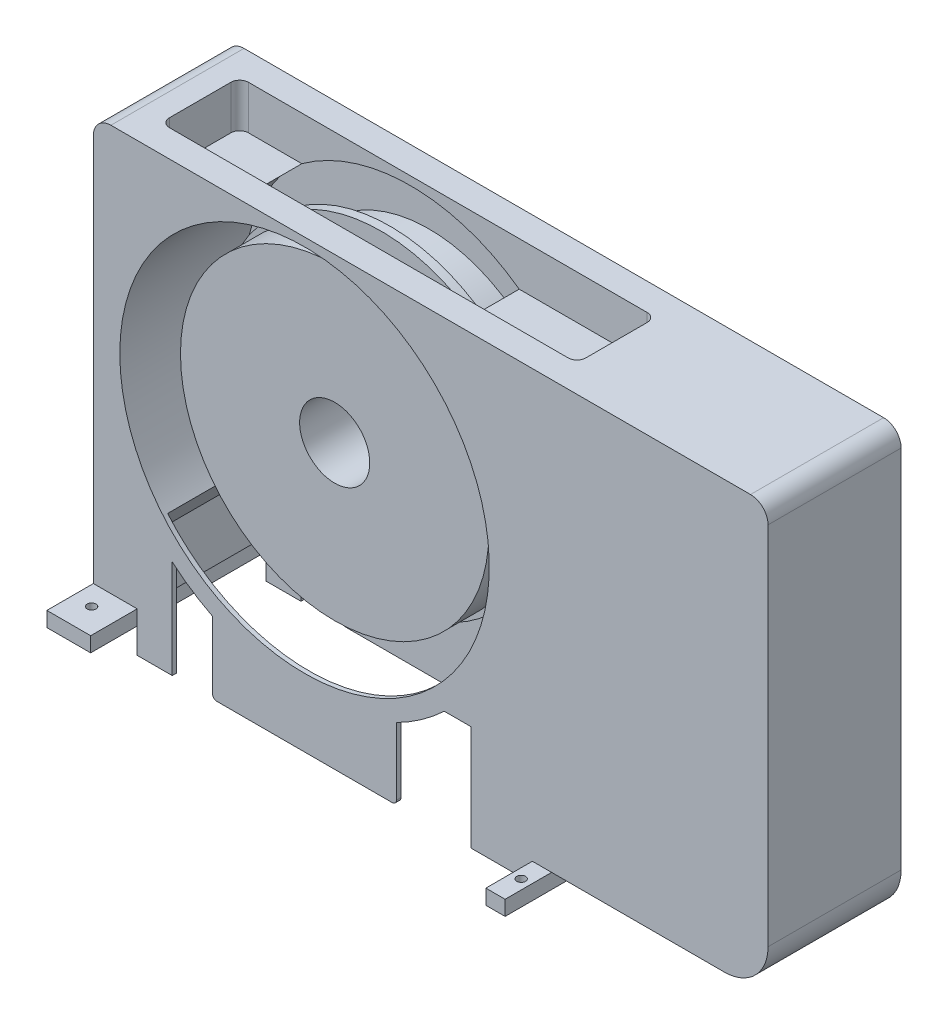
from build123d import *

# Parameters (mm, degrees)
SKETCH2_W             = 50
SKETCH2_H             = 17
BOSS_EXTRUDE1_DEPTH   = 205
SKETCH2_W_2           = 22
BOSS_EXTRUDE1_2_DEPTH = 205
SKETCH3_W             = 237
SKETCH3_H             = 453
BOSS_EXTRUDE2_DEPTH   = 151.9
BOSS_EXTRUDE3_DEPTH   = 10
SKETCH5_W             = 237
SKETCH5_H             = 453
BOSS_EXTRUDE4_DEPTH   = 5
SKETCH6_W             = 237
SKETCH6_H             = 453
BOSS_EXTRUDE5_DEPTH   = 5
BOSS_EXTRUDE7_DEPTH   = 5
BOSS_EXTRUDE8_DEPTH   = 5
BOSS_EXTRUDE9_DEPTH   = 5
FILLET1_R             = 20
FILLET2_R             = 50
CUT_EXTRUDE1_DEPTH    = 50
SKETCH13_W            = 50
SKETCH13_H            = 17
SKETCH13_W_2          = 22
BOSS_EXTRUDE10_DEPTH  = 30
SKETCH14_R            = 5
CUT_EXTRUDE2_DEPTH    = 742.238827909
SKETCH16_R            = 157.675
SKETCH16_R_2          = 52
BOSS_EXTRUDE12_DEPTH  = 54.4


with BuildPart() as part:
    # Sketch1 → Revolve1 (revolve)
    with BuildSketch(Plane(origin=(0, 318.5, 0), x_dir=(-1, 0, 0), z_dir=(0, -1, 0))):
        Polygon((-176, 125.5), (-167.675563156, 125.5), (-167.675563156, 120.5), (-157.675563156, 120.5), (-157.675563156, 140.5), (-182.675563156, 140.5), (-182.675563156, 150.5), (-40, 150.5), (-40, 87.5), (-176, 87.5), align=None)
    revolve(axis=Axis((0, 318.5, 0), (0, 0, -1)))



with BuildPart() as body_2:
    # Sketch2 → Boss-Extrude1 (new body)
    with BuildSketch(Plane.XY):
        with Locations((-216, 67.5)):
            Rectangle(SKETCH2_W, SKETCH2_H)
    extrude(amount=-BOSS_EXTRUDE1_DEPTH)



with BuildPart() as body_3:
    # Sketch2 → Boss-Extrude1 2 (new body)
    with BuildSketch(Plane.XY):
        with Locations((271, 43.5)):
            Rectangle(SKETCH2_W_2, SKETCH2_H)
    extrude(amount=-BOSS_EXTRUDE1_2_DEPTH)


with BuildPart() as body_2_1:
    add(body_2.part)

    add(body_3.part)  # Boss-Extrude2 merges body 3
    # Sketch3 → Boss-Extrude2 (add)
    with BuildSketch(Plane(origin=(0, 0, -53.1), x_dir=(-1, 0, 0), z_dir=(0, 0, -1))):
        with BuildLine():
            Line((-529, 539), (241, 539))
            Line((241, 539), (241, 76))
            Line((241, 76), (189.311768485, 76))
            Line((189.311768485, 76), (189.311768485, 143.562703206))
            Line((189.311768485, 143.562703206), (161.252096874, 182.66092141))
            ThreePointArc((161.252096874, 182.66092141), (32.69786622, 526.791487015), (-195.118401486, 238.604421776))
            Line((-195.118401486, 238.604421776), (-260, 205.941843226))
            Line((-260, 205.941843226), (-260, 52))
            Line((-260, 52), (-529, 52))
            Line((-529, 52), (-529, 539))
        make_face()
        with Locations((-400.5, 302.5)):
            Rectangle(SKETCH3_W, SKETCH3_H, mode=Mode.SUBTRACT)
        with BuildLine():
            Line((185.639383115, 174.406213053), (207.875695292, 143.422237275))
            ThreePointArc((207.875695292, 143.422237275), (219.062429829, 139.733284333), (226, 149.252818121))
            Line((226, 149.252818121), (226, 254.087268339))
            ThreePointArc((226, 254.087268339), (209.640199093, 212.311549949), (185.639383115, 174.406213053))
        make_face(mode=Mode.SUBTRACT)
    extrude(amount=BOSS_EXTRUDE2_DEPTH)

    # Sketch4 → Boss-Extrude3 (add)
    with BuildSketch(Plane(origin=(0, 0, -205), x_dir=(-1, 0, 0), z_dir=(0, 0, -1))):
        with BuildLine():
            Line((-196.910166335, 237.702414713), (-147.436524546, 262.608347182))
            ThreePointArc((-147.436524546, 262.608347182), (19.751163276, 474.933043742), (128.917329729, 227.716038197))
            Line((128.917329729, 227.716038197), (162.454726893, 180.985182237))
            ThreePointArc((162.454726893, 180.985182237), (33.181402046, 528.740000839), (-196.910166335, 237.702414713))
        make_face()
    extrude(amount=-BOSS_EXTRUDE3_DEPTH)

    # Sketch5 → Boss-Extrude4 (add)
    with BuildSketch(Plane(origin=(0, 0, -205), x_dir=(-1, 0, 0), z_dir=(0, 0, -1))):
        with Locations((-400.5, 302.5)):
            Rectangle(SKETCH5_W, SKETCH5_H)
    extrude(amount=-BOSS_EXTRUDE4_DEPTH)

    # Sketch6 → Boss-Extrude5 (add)
    with BuildSketch(Plane.XY.offset(-53.1)):
        with Locations((400.5, 302.5)):
            Rectangle(SKETCH6_W, SKETCH6_H)
    extrude(amount=-BOSS_EXTRUDE5_DEPTH)

    # Sketch8 → Boss-Extrude7 (add)
    with BuildSketch(Plane(origin=(0, 0, -205), x_dir=(-1, 0, 0), z_dir=(0, 0, -1))):
        with BuildLine():
            Line((-190, 30), (-190, 150))
            Line((-190, 150), (-120, 150))
            Line((-120, 150), (-105, 135))
            Line((-105, 135), (-105, 35))
            ThreePointArc((-105, 35), (-103.535533906, 31.464466094), (-100, 30))
            Line((-100, 30), (100, 30))
            ThreePointArc((100, 30), (103.535533906, 31.464466094), (105, 35))
            Line((105, 35), (105, 135))
            Line((105, 135), (120, 150))
            Line((120, 150), (151, 150))
            Line((151, 150), (151, 30))
            Line((151, 30), (191, 30))
            Line((191, 30), (191, 59))
            Line((191, 59), (191, 76))
            Line((191, 76), (189.311768485, 76))
            Line((189.311768485, 76), (189.311768485, 143.562703206))
            Line((189.311768485, 143.562703206), (129.750126988, 226.555622302))
            ThreePointArc((129.750126988, 226.555622302), (-20.083116117, 160.748510338), (-148.64860156, 261.998165534))
            Line((-148.64860156, 261.998165534), (-260, 205.941843226))
            Line((-260, 205.941843226), (-260, 30))
            Line((-260, 30), (-190, 30))
        make_face()
    extrude(amount=-BOSS_EXTRUDE7_DEPTH)

    # Sketch9 → Boss-Extrude8 (add)
    with BuildSketch(Plane.XY.offset(-53.1)):
        with BuildLine():
            Line((-185.639383115, 174.406213053), (-207.875695292, 143.422237275))
            ThreePointArc((-207.875695292, 143.422237275), (-219.062429829, 139.733284333), (-226, 149.252818121))
            Line((-226, 149.252818121), (-226, 254.087268339))
            ThreePointArc((-226, 254.087268339), (-209.640199093, 212.311549949), (-185.639383115, 174.406213053))
        make_face()
        with BuildLine():
            Line((-189.311768485, 143.562703206), (-189.311768485, 76))
            Line((-189.311768485, 76), (-191, 76))
            Line((-191, 76), (-191, 30))
            Line((-191, 30), (-151, 30))
            Line((-151, 30), (-151, 142.366527883))
            ThreePointArc((-151, 142.366527883), (-128.919838736, 125.617457554), (-105, 111.6208082))
            Line((-105, 111.6208082), (-105, 35))
            ThreePointArc((-105, 35), (-103.535533906, 31.464466094), (-100, 30))
            Line((-100, 30), (100, 30))
            ThreePointArc((100, 30), (103.535533906, 31.464466094), (105, 35))
            Line((105, 35), (105, 111.6208082))
            ThreePointArc((105, 111.6208082), (133.621776186, 128.844467708), (159.473352006, 150))
            Line((159.473352006, 150), (190, 150))
            Line((190, 150), (190, 30))
            Line((190, 30), (260, 30))
            Line((260, 30), (260, 35))
            Line((260, 35), (260, 52))
            Line((260, 52), (260, 205.941843226))
            Line((260, 205.941843226), (195.118401486, 238.604421776))
            ThreePointArc((195.118401486, 238.604421776), (32.69786622, 110.208512985), (-161.252096874, 182.66092141))
            Line((-161.252096874, 182.66092141), (-189.311768485, 143.562703206))
        make_face()
    extrude(amount=-BOSS_EXTRUDE8_DEPTH)

    # Sketch10 → Boss-Extrude9 (add)
    with BuildSketch(Plane(origin=(0, 0, -205), x_dir=(-1, 0, 0), z_dir=(0, 0, -1))):
        with BuildLine():
            Line((226, 149.252818121), (226, 254.087268339))
            ThreePointArc((226, 254.087268339), (209.640199093, 212.311549949), (185.639383115, 174.406213053))
            Line((185.639383115, 174.406213053), (207.875695292, 143.422237275))
            ThreePointArc((207.875695292, 143.422237275), (219.062429829, 139.733284333), (226, 149.252818121))
        make_face()
    extrude(amount=-BOSS_EXTRUDE9_DEPTH)

    # Fillet1
    fillet1_edges = [body_2_1.edges().sort_by_distance(p)[0] for p in [
        (-241, 539, -129.05),
        (529, 539, -129.05),
    ]]
    fillet(fillet1_edges, radius=FILLET1_R)

    # Fillet2
    fillet2_edges = [body_2_1.edges().sort_by_distance(p)[0] for p in [
        (529, 52, -129.05),
    ]]
    fillet(fillet2_edges, radius=FILLET2_R)

    # Sketch12 → Cut-Extrude1 (cut)
    with BuildSketch(Plane(origin=(0, 539, 0), x_dir=(1, 0, 0), z_dir=(0, 1, 0))):
        with BuildLine():
            Line((-185, 174.05), (270, 174.05))
            ThreePointArc((270, 174.05), (277.071067812, 171.121067812), (280, 164.05))
            Line((280, 164.05), (280, 94.05))
            ThreePointArc((280, 94.05), (277.071067812, 86.978932188), (270, 84.05))
            Line((270, 84.05), (-185, 84.05))
            ThreePointArc((-185, 84.05), (-192.071067812, 86.978932188), (-195, 94.05))
            Line((-195, 94.05), (-195, 164.05))
            ThreePointArc((-195, 164.05), (-192.071067812, 171.121067812), (-185, 174.05))
        make_face()
    extrude(amount=-CUT_EXTRUDE1_DEPTH, mode=Mode.SUBTRACT)

    # Sketch13 → Boss-Extrude10 (add)
    with BuildSketch(Plane(origin=(0, 0, -205), x_dir=(-1, 0, 0), z_dir=(0, 0, -1))):
        with Locations((216, 67.5)):
            Rectangle(SKETCH13_W, SKETCH13_H)
        with Locations((-271, 43.5)):
            Rectangle(SKETCH13_W_2, SKETCH13_H)
    extrude(amount=BOSS_EXTRUDE10_DEPTH)

    # Sketch14 → Cut-Extrude2 (cut, through all)
    with BuildSketch(Plane(origin=(0, 76, 0), x_dir=(1, 0, 0), z_dir=(0, 1, 0))):
        with Locations(Location((-219.303225542, 219.998090208, 0), (0, 0, 180))):
            Circle(SKETCH14_R)
        with Locations(Location((-219.303225542, 29.3636836, 0), (0, 0, 180))):
            Circle(SKETCH14_R)
        with Locations(Location((271, 219.998090208, 0), (0, 0, 90))):
            Circle(SKETCH14_R)
        with Locations(Location((271, 29.3636836, 0), (0, 0, 180))):
            Circle(SKETCH14_R)
    extrude(amount=-CUT_EXTRUDE2_DEPTH, mode=Mode.SUBTRACT)


with BuildPart() as part_1:
    add(part.part)

    add(body_2_1.part)  # Boss-Extrude12 merges body 2
    # Sketch16 → Boss-Extrude12 (add)
    with BuildSketch(Plane(origin=(0, 0, -150.5), x_dir=(-1, 0, 0), z_dir=(0, 0, -1))):
        with Locations(Location((0, 318.5, 0), (0, 0, 200.761196854))):
            Circle(SKETCH16_R)
        with Locations((0, 318.5)):
            Circle(SKETCH16_R_2, mode=Mode.SUBTRACT)
    extrude(amount=BOSS_EXTRUDE12_DEPTH)


solid = part_1.part
